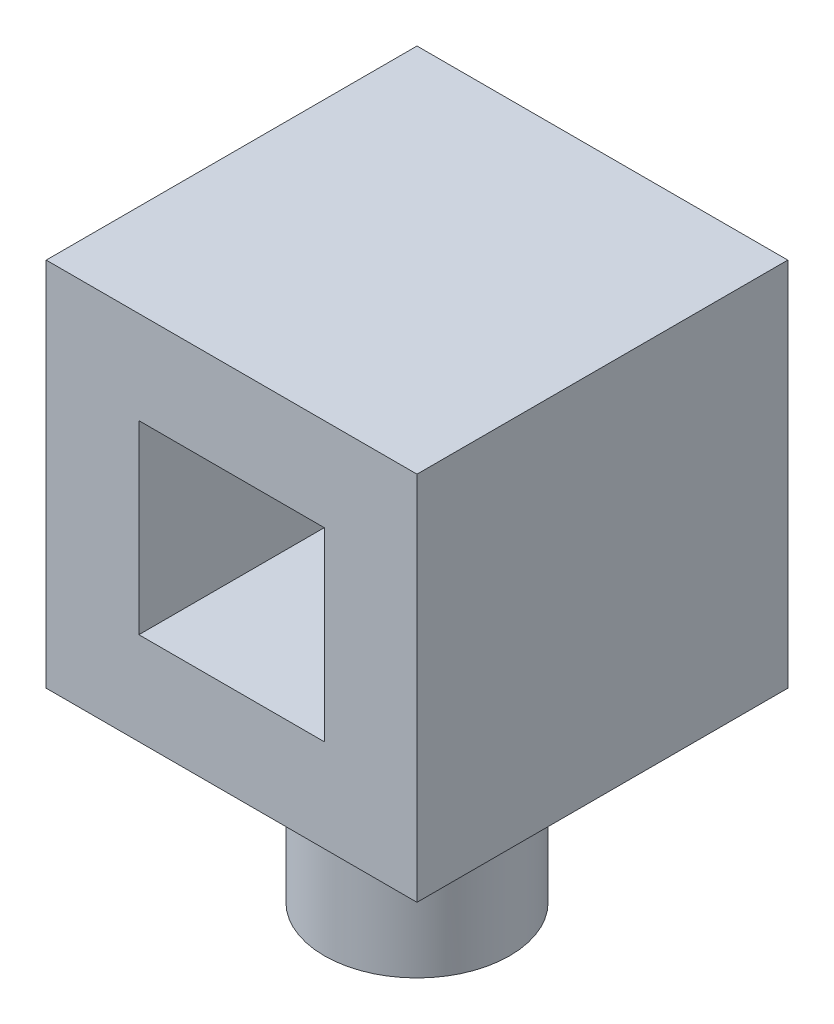
SolidWorks part; units mm, degrees
ref_plane "前视基准面" through (0, 0, 0) normal (0, 0, 1) x (1, 0, 0)
ref_plane "上视基准面" through (0, 0, 0) normal (0, 1, 0) x (1, 0, 0)
ref_plane "右视基准面" through (0, 0, 0) normal (1, 0, 0) x (0, 0, -1)
sketch "草图1" plane through (0, 0, 0) normal (0, 0, 1) x (1, 0, 0)
  line L1 (0, 0) -> (10, 0)
  line L2 (0, 0) -> (0, 10)
  line L3 (0, 10) -> (10, 10)
  line L4 (10, 0) -> (10, 10)
  line L5 (-5, -5) -> (15, -5)
  line L6 (-5, -5) -> (-5, 15)
  line L7 (-5, 15) -> (15, 15)
  line L8 (15, -5) -> (15, 15)
  dimension "D1" = 5
  dimension "D2" = 5
  dimension "D3" = 5
  dimension "D4" = 5
  dimension "D5" = 10
extrude "凸台-拉伸1" add sketch "草图1" along normal mid plane 20
sketch "草图2" plane through (0, -5, 0) normal (0, -1, 0) x (1, 0, 0)
  circle A0 centre (5, 0) radius 5
extrude "凸台-拉伸2" add sketch "草图2" along normal blind 10
